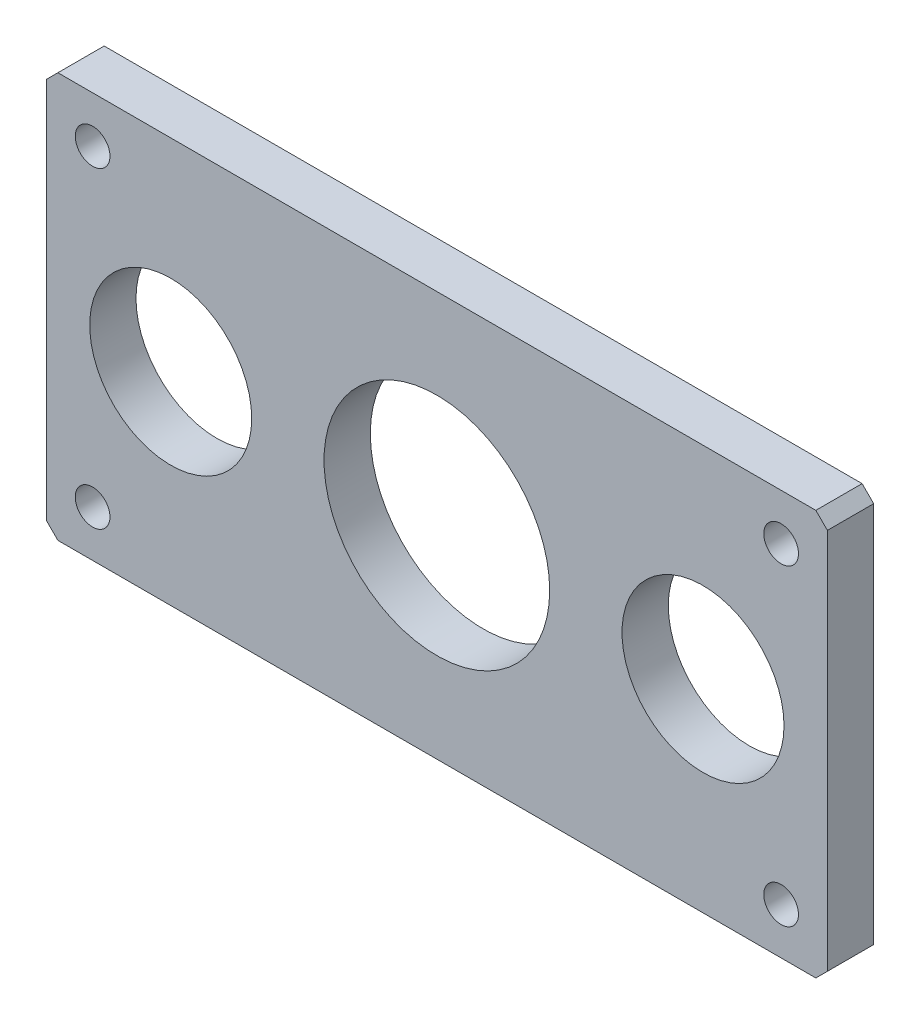
SolidWorks part; units mm, degrees
ref_plane "前视基准面" through (0, 0, 0) normal (0, 0, 1) x (1, 0, 0)
ref_plane "上视基准面" through (0, 0, 0) normal (0, 1, 0) x (1, 0, 0)
ref_plane "右视基准面" through (0, 0, 0) normal (1, 0, 0) x (0, 0, -1)
sketch "草图1" plane through (0, 0, 0) normal (0, 0, 1) x (1, 0, 0)
  line L1 (-67.5, -35) -> (67.5, -35)
  line L2 (-67.5, -35) -> (-67.5, 35)
  line L3 (-67.5, 35) -> (67.5, 35)
  line L4 (67.5, -35) -> (67.5, 35)
  line L5 (-67.5, -35) -> (67.5, 35) construction
  line L6 (-67.5, 35) -> (67.5, -35) construction
  point P0 (0, 0)
  dimension "D1" = 70
  dimension "D2" = 135
extrude "凸台-拉伸1" add sketch "草图1" along normal blind 8
sketch "草图2" plane through (0, 0, 8) normal (0, 0, 1) x (1, 0, 0)
  circle A0 centre (0, 0) radius 19.5
  dimension "D1" = 39
extrude "切除-拉伸1" cut sketch "草图2" against normal up to next
sketch "草图3" plane through (0, 0, 8) normal (0, 0, 1) x (1, 0, 0)
  line L0 (67.5, -35) -> (67.5, 35) construction
  line L1 (-67.5, 35) -> (-67.5, -35) construction
  circle A0 centre (46, 0) radius 14
  circle A1 centre (-46, 0) radius 14
extrude "切除-拉伸2" cut sketch "草图3" against normal up to next
sketch "草图4" plane through (0, 0, 8) normal (0, 0, 1) x (1, 0, 0)
  line L0 (67.5, 35) -> (-67.5, 35) construction
  line L1 (-67.5, 35) -> (-67.5, -35) construction
  line L2 (-67.5, -35) -> (67.5, -35) construction
  line L3 (0, 35) -> (0, -35) construction
  circle A0 centre (-59.5, 27) radius 3
  circle A1 centre (-59.5, -27) radius 3
  circle A2 centre (59.5, -27) radius 3
  circle A3 centre (59.5, 27) radius 3
  dimension "D1" = 6
  dimension "D2" = 8
  dimension "D3" = 8
  dimension "D4" = 8
extrude "切除-拉伸3" cut sketch "草图4" against normal up to next
chamfer "倒角1" distance 2 angle 45 4 edges at (-67.5, -35, 4) (67.5, -35, 4) (67.5, 35, 4) (-67.5, 35, 4)
equation "\"D3@草图3\"=\"D2@草图3\""
